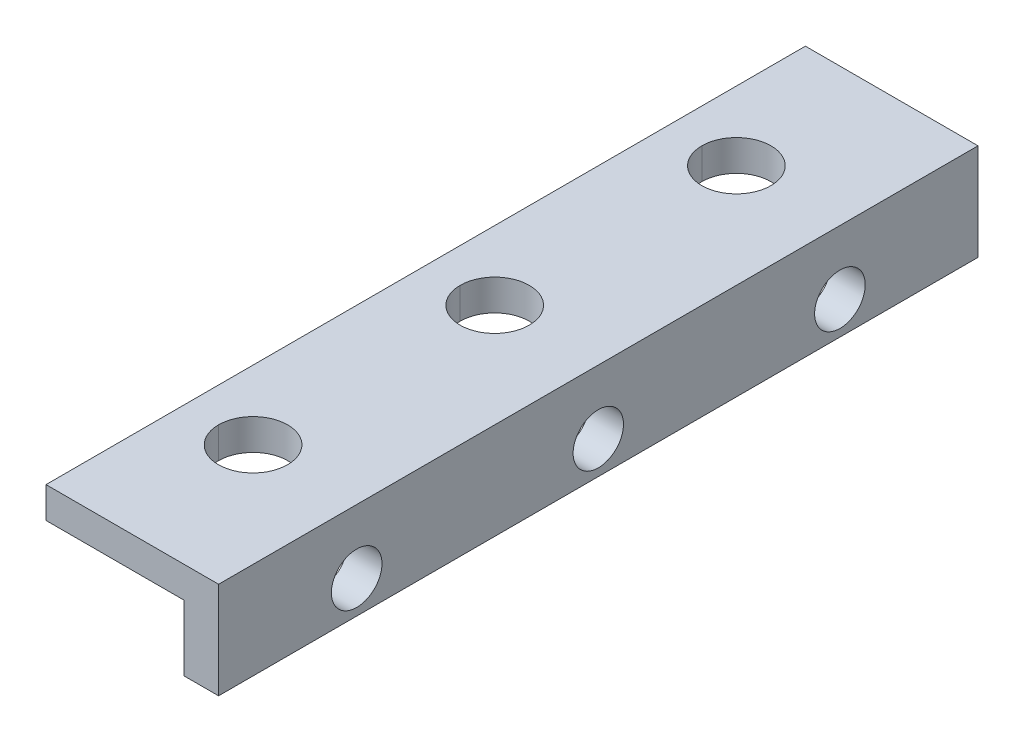
SolidWorks part; units mm, degrees
ref_plane "前视基准面" through (0, 0, 0) normal (0, 0, 1) x (1, 0, 0)
ref_plane "上视基准面" through (0, 0, 0) normal (0, 1, 0) x (1, 0, 0)
ref_plane "右视基准面" through (0, 0, 0) normal (1, 0, 0) x (0, 0, -1)
sketch "草图1" plane through (0, 0, 0) normal (0, 0, 1) x (1, 0, 0)
  line L0 (-55.5556, 26.25) -> (-5.5556, 26.25)
  line L1 (-5.5556, 26.25) -> (-5.5556, -1.75)
  line L2 (-5.5556, -1.75) -> (-15.5556, -1.75)
  line L3 (-15.5556, -1.75) -> (-15.5556, 17.25)
  line L4 (-15.5556, 17.25) -> (-55.5556, 17.25)
  line L5 (-55.5556, 26.25) -> (-55.5556, 17.25)
  dimension "D1" = 10
  dimension "D2" = 9
  dimension "D3" = 50
  dimension "D4" = 28
extrude "凸台-拉伸1" add sketch "草图1" along normal blind 220
extrude "切除-拉伸1" cut sketch "草图2" against normal up to surface (24 mm away)
sketch "草图2" plane through (982.7922, 17.25, -600.1263) normal (0, -1, 0) x (0.9997, 0, 0.0228)
  circle A0 centre (-1000.3032, 803.1683) radius 10
  circle A1 centre (-1001.8989, 733.1683) radius 10
  circle A2 centre (-1003.4947, 663.1683) radius 10
  circle A3 centre (-915.3257, 801.213) radius 10
  circle A4 centre (-916.9214, 731.213) radius 10
  circle A5 centre (-918.5167, 661.2312) radius 10
extrude "切除-拉伸2" cut sketch "草图3" against normal up to surface (24 mm away)
sketch "草图3" plane through (-968.9033, 17.25, 820.1263) normal (0, -1, 0) x (-0.9997, 0, -0.0228)
  circle A0 centre (-1000.3032, 803.1683) radius 10
  circle A1 centre (-1001.8989, 733.1683) radius 10
  circle A2 centre (-1003.4947, 663.1683) radius 10
  circle A3 centre (-915.3257, 801.213) radius 10
  circle A4 centre (-916.9214, 731.213) radius 10
  circle A5 centre (-918.5167, 661.2312) radius 10
extrude "切除-拉伸3" cut sketch "草图4" against normal up to surface (10 mm away) up to face at (-5.5556, 12.25, 110)
sketch "草图4" plane through (-15.5556, -796.8925, -600.1263) normal (-1, 0, 0) x (0, -1, 0)
  circle A0 centre (-804.6425, 640.1263) radius 7.3329
  circle A1 centre (-804.6425, 710.1263) radius 7.3013
  circle A2 centre (-804.6425, 780.1263) radius 6.6032
extrude "切除-拉伸4" cut sketch "草图5" against normal up to surface (45 mm away) up to face at (-15.5556, 7.75, 47.3329)
sketch "草图5" plane through (29.4444, -796.8925, 820.1263) normal (1, 0, 0) x (0, -1, 0)
  circle A0 centre (-804.6425, 640.1263) radius 7.3329
  circle A1 centre (-804.6425, 710.1263) radius 7.3013
  circle A2 centre (-804.6425, 780.1263) radius 6.6032
